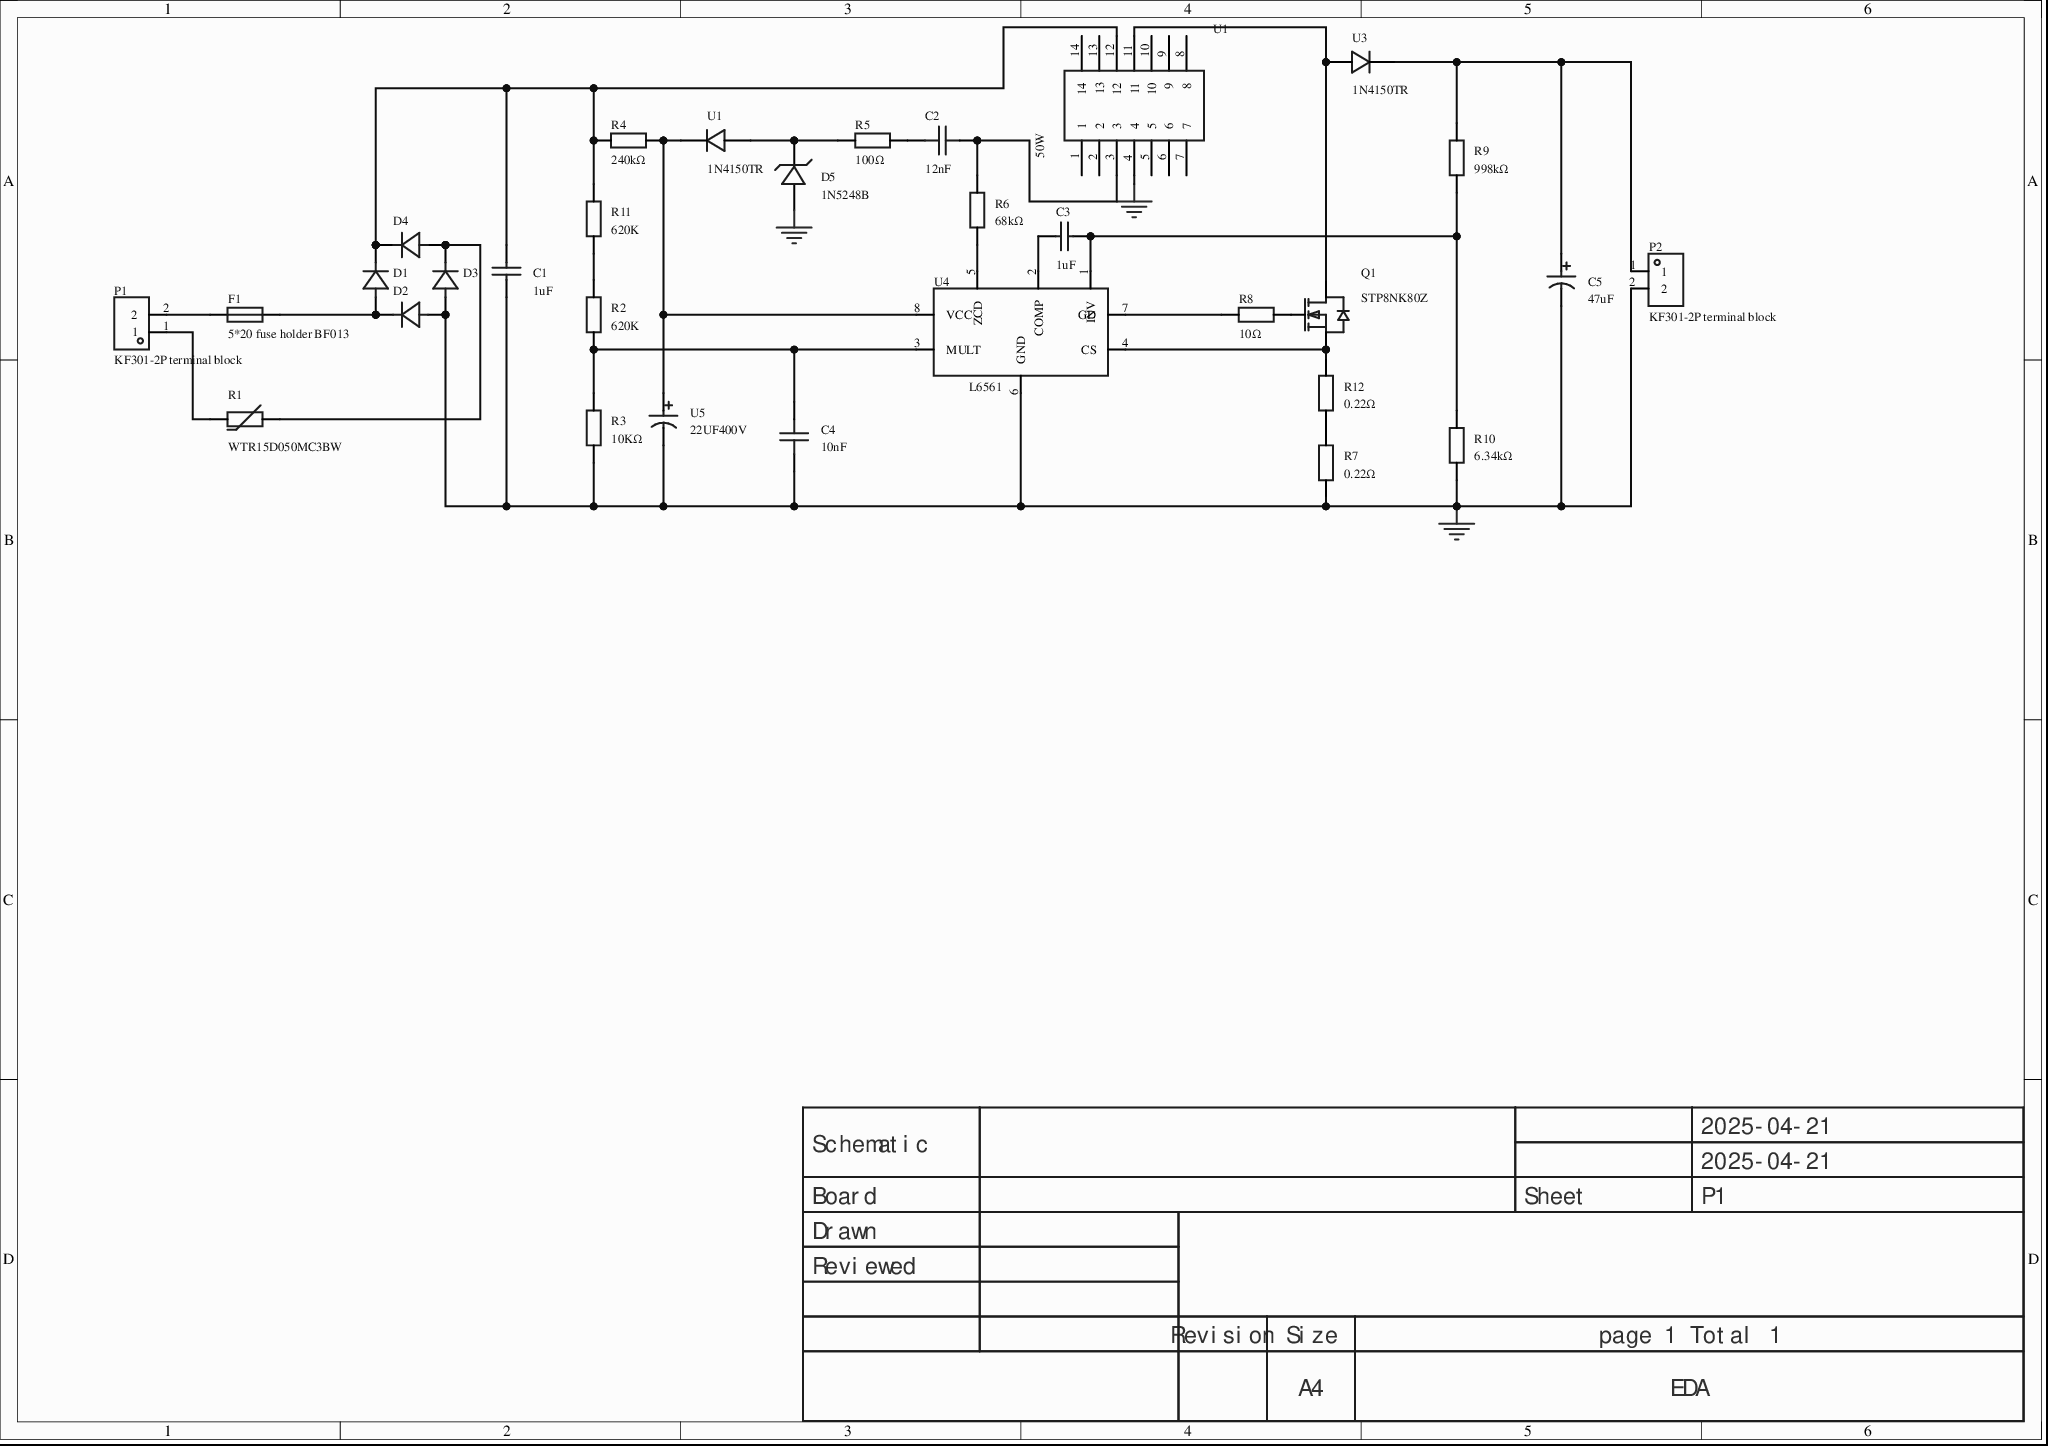
[diagram p0: MISC89005-3.schdoc]
# Altium project MISC89005-2.PrjPcb
1 sheet, 31 parts. Net scope: global (net labels, ports and power ports of the same name join across sheets).
Board file: MISC89005.pcbdoc

## Sheet MISC89005-3.schdoc
size 297 x 209 mm; Version: V1.0; @Project Name: MISC89005; @Page Count: 1; @Update Date: 2025-04-21; @Create Date: 2025-04-21; @Schematic Name: MISC89005; @Page No: 1; @Create Time: 19:10:21; @Update Time: 17:03:46; @Board Name: MISC89005

### Parts
(Parts that share a designator on the sheet are numbered #1, #2 ... from top to bottom, then left to right.)
C1  1uF  [CAP-TH_L18.0-W12.0-P15.00-D1.2]
C2  12nF  [CAP-TH_L7.3-W4.0-P5.00-D0.5]
C3  1uF  [CAP-TH_L18.0-W12.0-P15.00-D1.2]
C4  10nF  [CAP-TH_L5.5-W3.5-P5.00-D1.2]
C5  47uF  [CAP-TH_BD12.5-P5.00-D0.6-FD]
D1  (no value)  [DO_1N4007]
D2  (no value)  [DO_1N4007]
D3  (no value)  [DO_1N4007]
D4  (no value)  [DO_1N4007]
D5  1N5248B  [DO-35_BD2.0-L4.2-P8.20-D0.5-RD]
F1  5*20 fuse holder BF013  [FUSE-TH_BF013]
P1  KF301-2P terminal block  [CONN-TH_XY301V-A-5.0-2P]
P2  KF301-2P terminal block  [CONN-TH_XY301V-A-5.0-2P]
Q1  STP8NK80Z  [TO-220-3_L10.0-W4.5-P2.54-L]
R1  WTR15D050MC3BW  [RES-TH_L17.5-W6.0-P7.50-D0.8-S5.20]
R2  620K  [Res_1/4W]
R3  10KΩ  [Res_1/4W]
R4  240kΩ  [Res_1/4W]
R5  100Ω  [Res_1/4W]
R6  68kΩ  [Res_1/4W]
R7  0.22Ω  [Res_1W]
R8  10Ω  [Res_1/4W]
R9  998kΩ  [Res_1/4W]
R10  6.34kΩ  [Res_1/4W]
R11  620K  [Res_1/4W]
R12  0.22Ω  [Res_1W]
U1#1  1N4150TR  [DO-35_BD1.8-L4.1-P7.00-D0.5-RD]
U1#2  (no value)  [ETD29 卧式 14脚封装]
U3  1N4150TR  [DO-35_BD1.8-L4.1-P7.00-D0.5-RD]
U4  L6561  [DIP-8_L9.8-W6.6-P2.54-LS7.6-BL]
U5  22UF400V  [CAP-TH_BD8.0-P3.50-D0.6-FD]

### Nets
GND: C1.1 C4.1 C5.2 D2.2(A) D3.2(A) D5.2(A) P2.2 R3.1 R7.1 R10.2 U1#2.4 U4.6(GND) U5.2
NetC1_2: C1.2 D1.1(K) D4.1(K) R4.2 R11.2 U1#2.12
NetC2_1: C2.1 R5.1
NetC2_2: C2.2 R6.1 U1#2.3
NetC3_1: C3.1 R9.2 R10.1 U4.1(INV)
NetC3_2: C3.2 U4.2(COMP)
NetC4_2: C4.2 R2.1 R3.2 U4.3(MULT)
NetC5_1: C5.1 P2.1 R9.1 U3.1(K)
NetD1_2: D1.2(A) D2.1(K) F1.2
NetD3_1: D3.1(K) D4.2(A) R1.2
NetD5_1: D5.1(K) R5.2 U1#1.2(A)
NetF1_1: F1.1 P1.2
NetP1_1: P1.1 R1.1
NetQ1_1: Q1.1(G) R8.2
NetQ1_2: Q1.2(D) U1#2.11 U3.2(A)
NetQ1_3: Q1.3(S) R12.2 U4.4(CS)
NetR2_2: R2.2 R11.1
NetR4_1: R4.1 U1#1.1(K) U4.8(VCC) U5.1
NetR6_2: R6.2 U4.5(ZCD)
NetR7_2: R7.2 R12.1
NetR8_1: R8.1 U4.7(GD)

Not connected (* = marked no-connect by the designer): U1#2 1 2 5 6 7 8 9 10 13 14

### Notes on the sheet
- 2025-04-21
- Schematic
- Board
- Sheet
- P1
- Drawn
- Reviewed
- Revision
- Size
- A4
- page 1 Total 1
- EDA

### Library data of the parts
C1 C3 = MPP105K2W1912208LC: Capacitance:1uF;Tolerance:±10%;Rated voltage:450V;Operating temperature:-40℃~+85℃;; Manufacturer: SRD(圣融达); Symbol: MPP105K5191220LC; AddInBom: yes; ModelId: 3b36598c27314a5098d0bd2218fc3dd8; ModelName: CAP-TH_L17.5-W11.1-H14.3-P15.0; ModelTransform: 688.975,437.007,0,0,0,0,0,0,-137.795; Tolerance: ±10%; Voltage Rated: 450V; Device: MPP105K2W1912208LC; LCSC Part Name: 1uF ±10% 450V; SupplierPart: C109561; ManufacturerPart: MPP105K2W1912208LC; Supplier Footprint: 插件; JLCPCB Part Class: Extended library; Datasheet: https://atta.szlcsc.com/upload/public/pdf/source/20190820/C412730_D7BCD9B1AADCF68DA4089841D58A28D3.pdf; Supplier: LCSC; ConvertToPcb: yes; FootprintName: CAP-TH_L18.0-W12.0-P15.00-D1.2; Value: 1uF; Operating Temperature: -40℃~+85℃
C2 = LX2A123JD1B0070065035EOX: Capacitance:12nF;Tolerance:±5%;Rated voltage:100V;Dielectric:Metallized polyester;Operating temperature:-40℃~+125℃;; Manufacturer: STE(松田); AddInBom: yes; ModelId: 19b907e3d3ef40eaae8192aa4b2e4d9c; ModelName: CAP-TH_L7.3-W4.0-H7.5-P5.0; ModelTransform: 287.401,157.48,0,0,0,0,0,0,-137.795; Tolerance: ±5%; Voltage Rated: 100V; Symbol: LX2A123JD1B0070065035EOX; Device: LX2A123JD1B0070065035EOX; LCSC Part Name: 12nF ±5% 100V; SupplierPart: C435302; ManufacturerPart: LX2A123JD1B0070065035EOX; Supplier Footprint: 插件,P=5mm; JLCPCB Part Class: Extended library; Datasheet: https://atta.szlcsc.com/upload/public/pdf/source/20191009/C435355_F5D9FCDFBCE117FD74356CBCD037BC46.pdf; Supplier: LCSC; ConvertToPcb: yes; FootprintName: CAP-TH_L7.3-W4.0-P5.00-D0.5; Value: 12nF; Dielectric Material: Metallized polyester; Operating Temperature: -40℃~+125℃
C4 = C322C103JDR5TA: Capacitance:10nF;Rated voltage:1kV;Temperature coefficient:X7R;; Manufacturer: KEMET(基美); AddInBom: yes; ModelId: ea48d5c4e0d946599a66212ad84625b6; ModelName: CAP-TH_BD5.5-W3.5-P5.0; ModelTransform: 221.31003,137.795,0,0,0,0,0,0,-137.795; Voltage Rated: 1kV; Temperature Coefficient: X7R; Symbol: C322C103JDR5TA; Device: C322C103JDR5TA; LCSC Part Name: 10nF 1kV; SupplierPart: C183562; ManufacturerPart: C322C103JDR5TA; Supplier Footprint: 插件,P=5.08mm; JLCPCB Part Class: Extended library; Datasheet: https://atta.szlcsc.com/upload/public/pdf/source/20180316/EDE9EE9FCEB6737093FCB1BAE58FB051.pdf; Supplier: LCSC; ConvertToPcb: yes; FootprintName: CAP-TH_L5.5-W3.5-P5.00-D1.2; Value: 10nF
C5 = KM476M200J20RR0VH2FP0: Capacitance:47uF;Tolerance:±20%;Rated voltage:200V;; Manufacturer: CX(承兴); Symbol: 47uf200v13*20mm; AddInBom: yes; ModelId: 968d8ff988964aab8919b46a6a737be2; ModelName: CAP-TH_D12.5-H20.0-P5.00; ModelTransform: 492.5187,492.11201,0,0,0,0,0,0,-137.795; Tolerance: ±20%; Voltage Rating: 200V; Pin Spacing: 5mm; Lifetime: 2000hrs@105℃; Device: KM476M200J20RR0VH2FP0; LCSC Part Name: 47uF ±20% 200V; SupplierPart: C33987; ManufacturerPart: KM476M200J20RR0VH2FP0; Supplier Footprint: 插件,D13xL20mm; JLCPCB Part Class: Extended library; Datasheet: https://atta.szlcsc.com/upload/public/pdf/source/20211027/06D6BA3719C264B639DC286D935D03EA.pdf; Supplier: LCSC; ConvertToPcb: yes; FootprintName: CAP-TH_BD12.5-P5.00-D0.6-FD; Value: 47uF; Diameter: 13mm; Height - Seated (Max): 20mm
D1-D4 = D_1N4007A: AddInBom: yes; ModelId: 6de1e9b71a0d4751b4e9df530304c1a3; ModelName: DO-41_D2.4-L4.7-P8.70; ModelTransform: 373.9,94.4,232.29,0,0,0,0,0,-140; Symbol: D_1N4007; Device: D_1N4007A; Supplier Footprint: DO-41; ConvertToPcb: yes; FootprintName: DO_1N4007
D5 = 1N5248B: Diode configuration:Single;Zener voltage(nominal):18V;Zener voltage(range):17.1V~18.9V;Power(Pd):500mW;; Manufacturer: ST(先科); AddInBom: yes; ModelId: 6e6fa891745c42b796728c269d94cdcf; ModelName: DO-35_D1.9-L3.9-P8.2; ModelTransform: 342.519,74.82103,0,0,0,0,-0.197,1.181,-137.795; Diode Configuration: Single; Zener Voltage (Nom): 18V; Reverse Leakage Current (Ir): 100nA@14V; Power Dissipation: 500mW; Zener Impedance (Zzt): 21Ω; Symbol: 1N5248B; Device: 1N5248B; LCSC Part Name: 1N5248B 停产 此料号已停产，后续升级为无铅玻璃料号1N5248BPF,升级产品性能品质不变; SupplierPart: C118667; ManufacturerPart: 1N5248B; Supplier Footprint: DO-35; JLCPCB Part Class: Extended library; Datasheet: https://atta.szlcsc.com/upload/public/pdf/source/20150124/1457707264094.pdf; Supplier: LCSC; ConvertToPcb: yes; FootprintName: DO-35_BD2.0-L4.2-P8.20-D0.5-RD; Zener Voltage (Range): 17.1V~18.9V
F1 = 5*20保险丝座BF013: AddInBom: yes; ModelId: b24d2030d84e43169d20d72a25ad3443; ModelTransform: 830.707,362.204,0,0,0,0,0,0,-157.48; Symbol: 5*20 fuse holder BF013; Device: 5*20 fuse holder BF013; LCSC Part Name: 5*20保险丝座BF013; SupplierPart: C9900020280; ManufacturerPart: 5*20保险丝座BF013; Supplier Footprint: P=15.3; JLCPCB Part Class: Extended library; Supplier: LCSC; ConvertToPcb: yes; FootprintName: FUSE-TH_BF013; ModelName: FUSE-TH_BF013
P1 P2 = KF301-2P接线端子: AddInBom: yes; ModelId: ef7ead88b0f2448d904975b26718870f; ModelTransform: 417.322,299.212,0,0,0,0,11.811,-7.835,-157.48; Symbol: KF301-2P terminal block; Device: KF301-2P terminal block; LCSC Part Name: KF301-2P接线端子; SupplierPart: C9900016950; ManufacturerPart: KF301-2P接线端子; Supplier Footprint: CK301-2P; JLCPCB Part Class: Extended library; Supplier: LCSC; ConvertToPcb: yes; FootprintName: CONN-TH_XY301V-A-5.0-2P; ModelName: CONN-TH_XY301V-A-5.0-2P
Q1 = STP8NK80Z: 类型:1个N沟道;漏源电压(Vdss):800V;连续漏极电流(Id):6.2A;功率(Pd):140W;导通电阻(RDS(on)@Vgs,Id):1.5Ω@10V,3.1A;阈值电压(Vgs(th)@Id):4.5V@100uA;; Manufacturer: ST(意法半导体); AddInBom: yes; ModelId: b3c9e38e4428458f8b925050989b538f; ModelTransform: 397.637,177.165,0,180,0,0,-0.004,19.88,-78.74; Type: 1 N-channel; Drain Source Voltage (Vdss): 800V; Continuous Drain Current (Id): 6.2A; Power Dissipation (Pd): 140W; Symbol: STP8NK80Z; Device: STP8NK80Z; LCSC Part Name: 1个N沟道 耐压:800V 电流:6.2A; SupplierPart: C472641; ManufacturerPart: STP8NK80Z; Supplier Footprint: TO-220; Datasheet: https://atta.szlcsc.com/upload/public/pdf/source/20191219/C472641_AB60B72FC5243B1EC67B7B4A11A44509.pdf; Supplier: LCSC; ConvertToPcb: yes; FootprintName: TO-220-3_L10.0-W4.5-P2.54-L; ModelName: TO-220-3_L10.0-W4.5-P2.54-L; Drain Source On Resistance (RDS(on)@Vgs,Id): 1.5Ω@10V,3.1A; Gate Threshold Voltage (Vgs(th)@Id): 4.5V@100uA
R1 = WTR15D050MC3BW: Resistance(25℃):-;Resistance tolerance:-;Max working voltage:-;Power:-;; Manufacturer: WMEC(万明); AddInBom: yes; ModelId: e68b4e892efa40d2a48ddeddecfa2b85; ModelName: RES-TH_L17.5-W6.0-P7.50-S5.20; ModelTransform: 688.39551,236.22,0,0,0,0,0,0,-137.795; Symbol: WTR15D050MC3BW; Device: WTR15D050MC3BW; LCSC Part Name: 热敏电阻 5欧 (5D-15) 停产; SupplierPart: C523875; ManufacturerPart: WTR15D050MC3BW; Supplier Footprint: 插件,P=7.5mm; JLCPCB Part Class: Extended library; Datasheet: https://atta.szlcsc.com/upload/public/pdf/source/20200428/C523875_85C4FDEE3F3521A14A711A7A31AE3BBE.pdf; Supplier: LCSC; ConvertToPcb: yes; FootprintName: RES-TH_L17.5-W6.0-P7.50-D0.8-S5.20; Resistance @ 25℃: -; Resistance Tolerance: -; Vmax: -; Operating Temperature: -; Power: -
R2-R6 R8-R11 = Res_AXIAL-1/4W: AddInBom: yes; SymbolName: Resistor; ModelId: 463263665006444ab7a47bd11b0cf956; ModelName: RES-TH_BD2.4-L6.3-P10.30-D0.6; ModelTransform: 427.165,94.32816,0,0,0,0,0,0,-196.85; Device: Res_AXIAL-1/4W; Supplier Footprint: 轴向引线; ConvertToPcb: yes; FootprintName: Res_1/4W
  R2 R11: Value: 620K
  R3: Value: 10KΩ
  R4: Value: 240kΩ
  R5: Value: 100Ω
  R6: Value: 68kΩ
  R8: Value: 10Ω
  R9: Value: 998kΩ
  R10: Value: 6.34kΩ
R7 R12 = Res_AXIAL-1W: ConvertToPcb: yes; SymbolName: Resistor; ModelId: f1f7cfb3d56f4763951150e77c261d09; ModelName: RES-TH_BD4.5-L11.5-P15.50-D0.8; ModelTransform: 641.71,177.16,374,0,0,0,0,0,-190; Value: 0.22Ω; Device: Res_AXIAL-1W; AddInBom: yes; Supplier Footprint: 轴向引线; FootprintName: Res_1W
U1#1 U3 = 1N4150TR: Diode configuration:Single;Forward voltage(Vf):1V@200mA;DC reverse voltage(Vr):50V;Rectified current:200mA;Reverse recovery time(trr):6ns;; Manufacturer: onsemi(安森美); AddInBom: yes; ModelId: ef533f79b9ab433ca3f5550a32d3a157; ModelTransform: 295.275,71.22773,0,0,0,0,0,0,-196.85; Diode Configuration: Single; Reverse Voltage (Vr): 50V; Rectified Current: 200mA; Reverse Leakage Current: 100nA@50V; Reverse Recovery Time (trr): 6ns; Symbol: 1N4150TR; Device: 1N4150TR; LCSC Part Name: 电压:50V 电流:200mA; SupplierPart: C3312787; ManufacturerPart: 1N4150TR; Supplier Footprint: DO-35; JLCPCB Part Class: Extended library; Datasheet: https://atta.szlcsc.com/upload/public/pdf/source/20230915/F5D719126421BDA0D8959E8DD4753432.pdf; Supplier: LCSC; ConvertToPcb: yes; FootprintName: DO-35_BD1.8-L4.1-P7.00-D0.5-RD; ModelName: DO-35_BD1.8-L4.1-P7.00-D0.5-RD; Forward Voltage (Vf@If): 1V@200mA; Operating Temperature: -
U1#2 = 50W-900-50-24-16-06: 50W DC900V 高压高频变压器，可输出24V 50W  正负16V  0.1A 6V 0.1A .独立正16V，也可输出2A  反馈回路最大可提供15W .但是总功率不要超过50W; Add into BOM: yes; Device: 50W-900-50-24-16-06; Convert to PCB: yes; SymbolName: 50W-900-50-24-16-06; FootprintName: ETD29 horizontal 14-pin package
U4 = L6561: Supply voltage:11V~18V;; Manufacturer: ST(意法半导体); AddInBom: yes; ModelId: db2af726fcec488f8bf8e467aca974b3; ModelName: DIP-8_L9.8-W6.6-H3.5-LS7.62-P2.54; ModelTransform: 385.826,311.8104,0,0,0,0,-1.693,0,-137.795; Symbol: L6561; Device: L6561; LCSC Part Name: L6561; SupplierPart: C361021; ManufacturerPart: L6561; Supplier Footprint: DIP-8; Datasheet: https://atta.szlcsc.com/upload/public/pdf/source/20150821/1457707348882.pdf; Supplier: LCSC; ConvertToPcb: yes; Supply Voltage: 11V~18V; Operating Temperature: -25℃~+125℃; FootprintName: DIP-8_L9.8-W6.6-P2.54-LS7.6-BL
U5 = 22UF400V: AddInBom: yes; ModelId: a2c936ec27754f809f3966430e36f767; ModelName: CAP-TH_D8.0-H8.0-P3.50; ModelTransform: 314.96,314.862,0,180,0,0,0,0,-137.795; Symbol: 22UF400V; Device: 22UF400V; LCSC Part Name: 22UF400V; SupplierPart: C9900013823; ManufacturerPart: 22UF400V; Supplier Footprint: 22uF400V; Supplier: LCSC; ConvertToPcb: yes; FootprintName: CAP-TH_BD8.0-P3.50-D0.6-FD